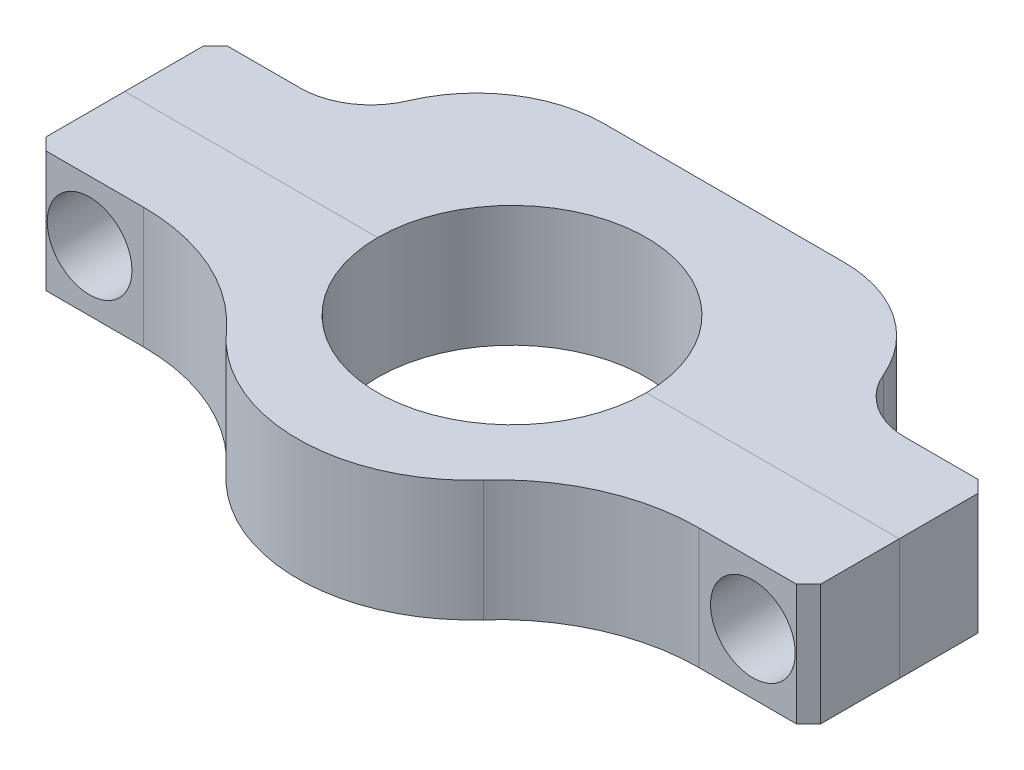
SolidWorks part; units mm, degrees
ref_plane "Front Plane" through (0, 0, 0) normal (0, 0, 1) x (1, 0, 0)
ref_plane "Top Plane" through (0, 0, 0) normal (0, 1, 0) x (1, 0, 0)
ref_plane "Right Plane" through (0, 0, 0) normal (1, 0, 0) x (0, 0, -1)
sketch "Sketch1" plane through (0, 0, 0) normal (0, 1, 0) x (1, 0, 0)
  line L0 (0, 21.1747) -> (0, -23.2296) construction
  line L1 (-26.6867, 0) -> (28.0913, 0) construction
  line L2 (9.9239, 12.7458) -> (-9.9239, 12.7458)
  line L3 (-25, 2.7458) -> (-32, 2.7458)
  line L4 (-32, 2.7458) -> (-32, -12.2542)
  line L5 (-32, -12.2542) -> (-22.9303, -12.2542)
  line L6 (32, -12.2542) -> (22.9303, -12.2542)
  line L7 (32, 2.7458) -> (32, -12.2542)
  line L8 (25, 2.7458) -> (32, 2.7458)
  arc A0 (-9.9239, 12.7458) -> (-19.6142, 6.3182) centre (-9.9239, 2.2274) ccw
  arc A1 (-19.6142, 6.3182) -> (-25, 2.7458) centre (-25, 8.5919) cw
  arc A2 (-22.9303, -12.2542) -> (-10.619, -17.7383) centre (-22.9303, -28.815) cw
  arc A3 (-10.619, -17.7383) -> (10.619, -17.7383) centre (0, -8.1841) ccw
  arc A4 (22.9303, -12.2542) -> (10.619, -17.7383) centre (22.9303, -28.815) ccw
  arc A5 (19.6142, 6.3182) -> (25, 2.7458) centre (25, 8.5919) ccw
  arc A6 (9.9239, 12.7458) -> (19.6142, 6.3182) centre (9.9239, 2.2274) cw
  point P27 (0, 12.7458)
  dimension "D1" = 64
  dimension "D2" = 10
  dimension "D3" = 15
  dimension "D4" = 7
extrude "Boss-Extrude1" add sketch "Sketch1" along normal blind 10
sketch "Sketch2" plane through (0, 10, 0) normal (0, 1, 0) x (1, 0, 0)
  line L0 (-32, -4.7542) -> (32, -4.7542)
  line L1 (-32, 2.7458) -> (-32, -12.2542) construction
  line L2 (32, 2.7458) -> (32, -12.2542) construction
split line "Split Line1"
chamfer "Chamfer1" distance 1 angle 45 4 edges at (-32, 5, 12.2542) (-32, 5, -2.7458) (32, 5, 12.2542) (32, 5, -2.7458)
sketch "Sketch3" plane through (0, 0, 0) normal (0, 0, 1) x (1, 0, 0)
  line L0 (0, 17.036) -> (0, -7.8849) construction
  circle A0 centre (27.4008, 5) radius 3.5
  circle A1 centre (-27.4008, 5) radius 3.5
  dimension "D1" = 7
extrude "Cut-Extrude1" cut sketch "Sketch3" along normal blind 20 from vertex at 4.7542
sketch "Sketch7" plane through (0, 10, 0) normal (0, 1, 0) x (1, 0, 0)
  line L0 (32, -4.7542) -> (-32, -4.7542) construction
  circle A0 centre (0, -4.7542) radius 11.1
  dimension "D1" = 22.2
extrude "Cut-Extrude2" cut sketch "Sketch7" against normal blind 20
